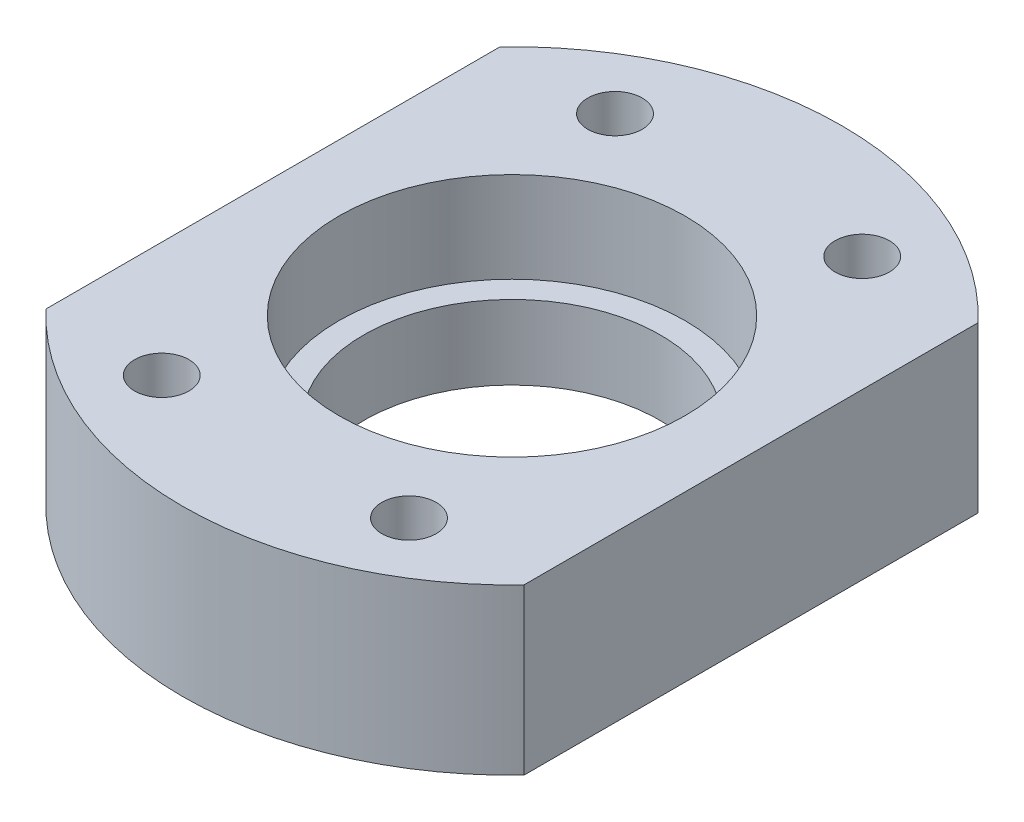
from build123d import *

# Parameters (mm, degrees)
SKETCH1_R                      = 40
BOSS_EXTRUDE1_DEPTH            = 20
SKETCH2_R                      = 21
CUT_EXTRUDE1_DEPTH             = 11
SKETCH3_R                      = 18
CUT_EXTRUDE2_DEPTH             = 11
CUT_EXTRUDE3_DEPTH             = 61
M6_CLEARANCE_HOLE2_D           = 6.6
M6_CLEARANCE_HOLE2_CSINK_D     = 6.65
M6_CLEARANCE_HOLE2_CSINK_ANGLE = 90


with BuildPart() as part:
    # Sketch1 → Boss-Extrude1 (new body)
    with BuildSketch(Plane(origin=(0, 0, 0), x_dir=(1, 0, 0), z_dir=(0, 1, 0))):
        with Locations(Location((0, 0, 0), (0, 0, 270))):
            Circle(SKETCH1_R)
    extrude(amount=BOSS_EXTRUDE1_DEPTH)

    # Sketch2 → Cut-Extrude1 (cut)
    with BuildSketch(Plane(origin=(0, 20, 0), x_dir=(1, 0, 0), z_dir=(0, 1, 0))):
        with Locations(Location((0, 0, 0), (0, 0, 270))):
            Circle(SKETCH2_R)
    extrude(amount=-CUT_EXTRUDE1_DEPTH, mode=Mode.SUBTRACT)

    # Sketch3 → Cut-Extrude2 (cut)
    with BuildSketch(Plane(origin=(0, 9, 0), x_dir=(1, 0, 0), z_dir=(0, 1, 0))):
        with Locations(Location((0, 0, 0), (0, 0, 270))):
            Circle(SKETCH3_R)
    extrude(amount=-CUT_EXTRUDE2_DEPTH, mode=Mode.SUBTRACT)

    # Sketch8 → Cut-Extrude3 (cut, through all)
    with BuildSketch(Plane.XZ):
        with BuildLine():
            ThreePointArc((40, 0), (37.148351242, 14.832396974), (29, 27.549954628))
            Line((29, 27.549954628), (29, -27.549954628))
            ThreePointArc((29, -27.549954628), (37.148351242, -14.832396974), (40, 0))
        make_face()
        with BuildLine():
            ThreePointArc((-29, 27.549954628), (-40, 0), (-29, -27.549954628))
            Line((-29, -27.549954628), (-29, 27.549954628))
        make_face()
    extrude(amount=-CUT_EXTRUDE3_DEPTH, mode=Mode.SUBTRACT)

    # M6 Clearance Hole2 (through all)
    with Locations(Plane(origin=(0, 0, 0), x_dir=(-1, 0, 0), z_dir=(0, -1, 0))):
        with Locations((-15, -27.5), (15, -27.5), (15, 27.5), (-15, 27.5)):
            CounterSinkHole(M6_CLEARANCE_HOLE2_D / 2, M6_CLEARANCE_HOLE2_CSINK_D / 2, counter_sink_angle=M6_CLEARANCE_HOLE2_CSINK_ANGLE)


solid = part.part
